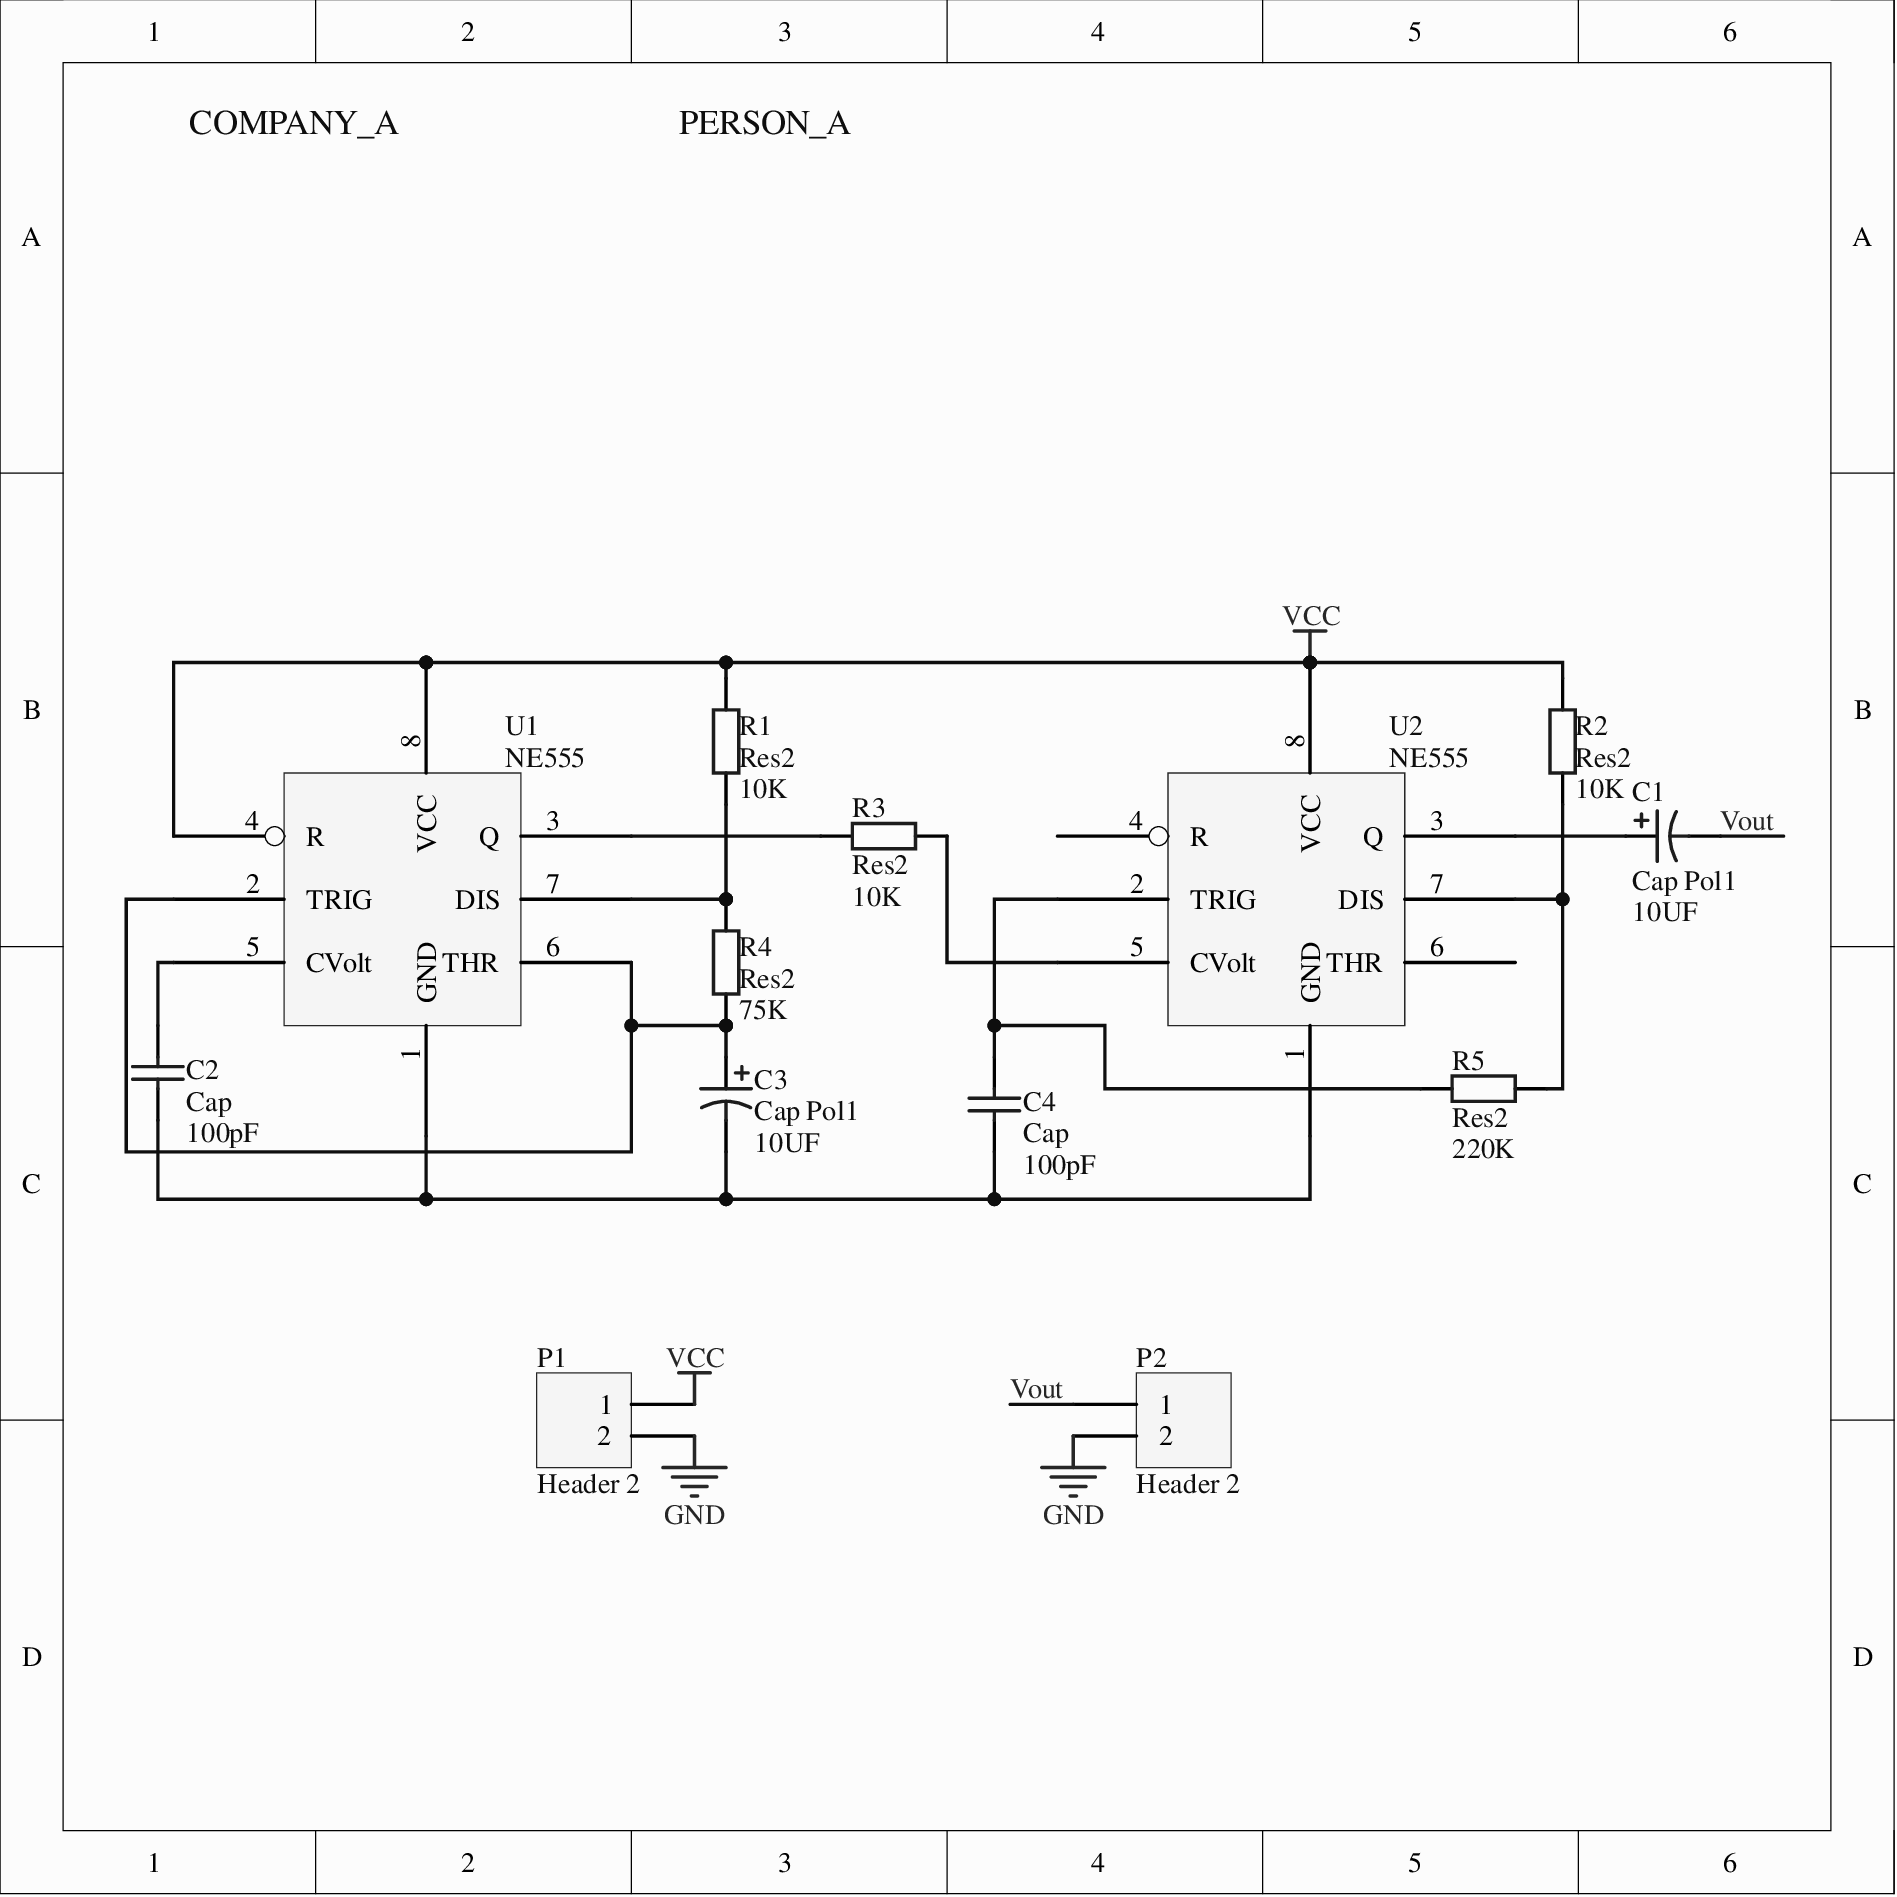
[diagram p0: MISC80651.SchDoc]
# Altium project MISC80651.PrjPcb
1 sheet, 13 parts. Net scope: global (net labels, ports and power ports of the same name join across sheets).
Board file: MISC80651.PcbDoc

## Sheet MISC80651.SchDoc
size 152 x 152 mm

### Parts
C1  Cap Pol1  value 10UF  [RB7.6-15]
C2  Cap  value 100pF  [RAD-0.3]
C3  Cap Pol1  value 10UF  [RB7.6-15]
C4  Cap  value 100pF  [RAD-0.3]
P1  Header 2  [HDR1X2]
P2  Header 2  [HDR1X2]
R1  Res2  value 10K  [AXIAL-0.4]
R2  Res2  value 10K  [AXIAL-0.4]
R3  Res2  value 10K  [AXIAL-0.4]
R4  Res2  value 75K  [AXIAL-0.4]
R5  Res2  value 220K  [AXIAL-0.4]
U1  NE555  [DIP8]
U2  NE555  [DIP8]

### Nets
GND: P1.2 P2.2
VCC: P1.1 R1.2 R2.2 U1.4(R) U1.8(VCC) U2.8(VCC)
Vout: C1.2 P2.1
NetC1_1: C1.1 U2.3(Q)
NetC2_1: C2.1 C3.2 C4.1 U1.1(GND) U2.1(GND)
NetC2_2: C2.2 U1.5(CVolt)
NetC3_1: C3.1 R4.1 U1.2(TRIG) U1.6(THR)
NetC4_2: C4.2 R5.2 U2.2(TRIG)
NetR1_1: R1.1 R4.2 U1.7(DIS)
NetR2_1: R2.1 R5.1 U2.7(DIS)
NetR3_1: R3.1 U2.5(CVolt)
NetR3_2: R3.2 U1.3(Q)

Not connected (* = marked no-connect by the designer): U2 4(R) 6(THR)

### Notes on the sheet
- COMPANY_A
- PERSON_A

### Library data of the parts
C1 C3 = Cap Pol1: Polarized Capacitor (Radial); Published: 8-Jun-2000; LatestRevisionDate: 17-Jul-2002; LatestRevisionNote: Re-released for DXP Platform.; PackageReference: RB7.6-15; PackageDescription: Polarized Capacitor (Radial); 2 Leads; Publisher: Altium Limited
C2 C4 = Cap: Capacitor; Published: 8-Jun-2000; LatestRevisionDate: 17-Jul-2002; LatestRevisionNote: Re-released for DXP Platform.; PackageReference: RAD-0.3; PackageDescription: Radial Cap, Thru-Hole; 2 Leads; 0.3 in Pin Spacing; Publisher: Altium Limited
P1 P2 = Header 2: Header, 2-Pin; LatestRevisionDate: 17-Jul-2002; LatestRevisionNote: Re-released for DXP Platform.; Publisher: Altium Limited
R1-R5 = Res2: Resistor; Published: 8-Jun-2000; LatestRevisionDate: 17-Jul-2002; LatestRevisionNote: Re-released for DXP Platform.; PackageReference: AXIAL-0.4; PackageDescription: Axial Device, Thru-Hole; 2 Leads; 0.4 in Pin Spacing; Publisher: Altium Limited